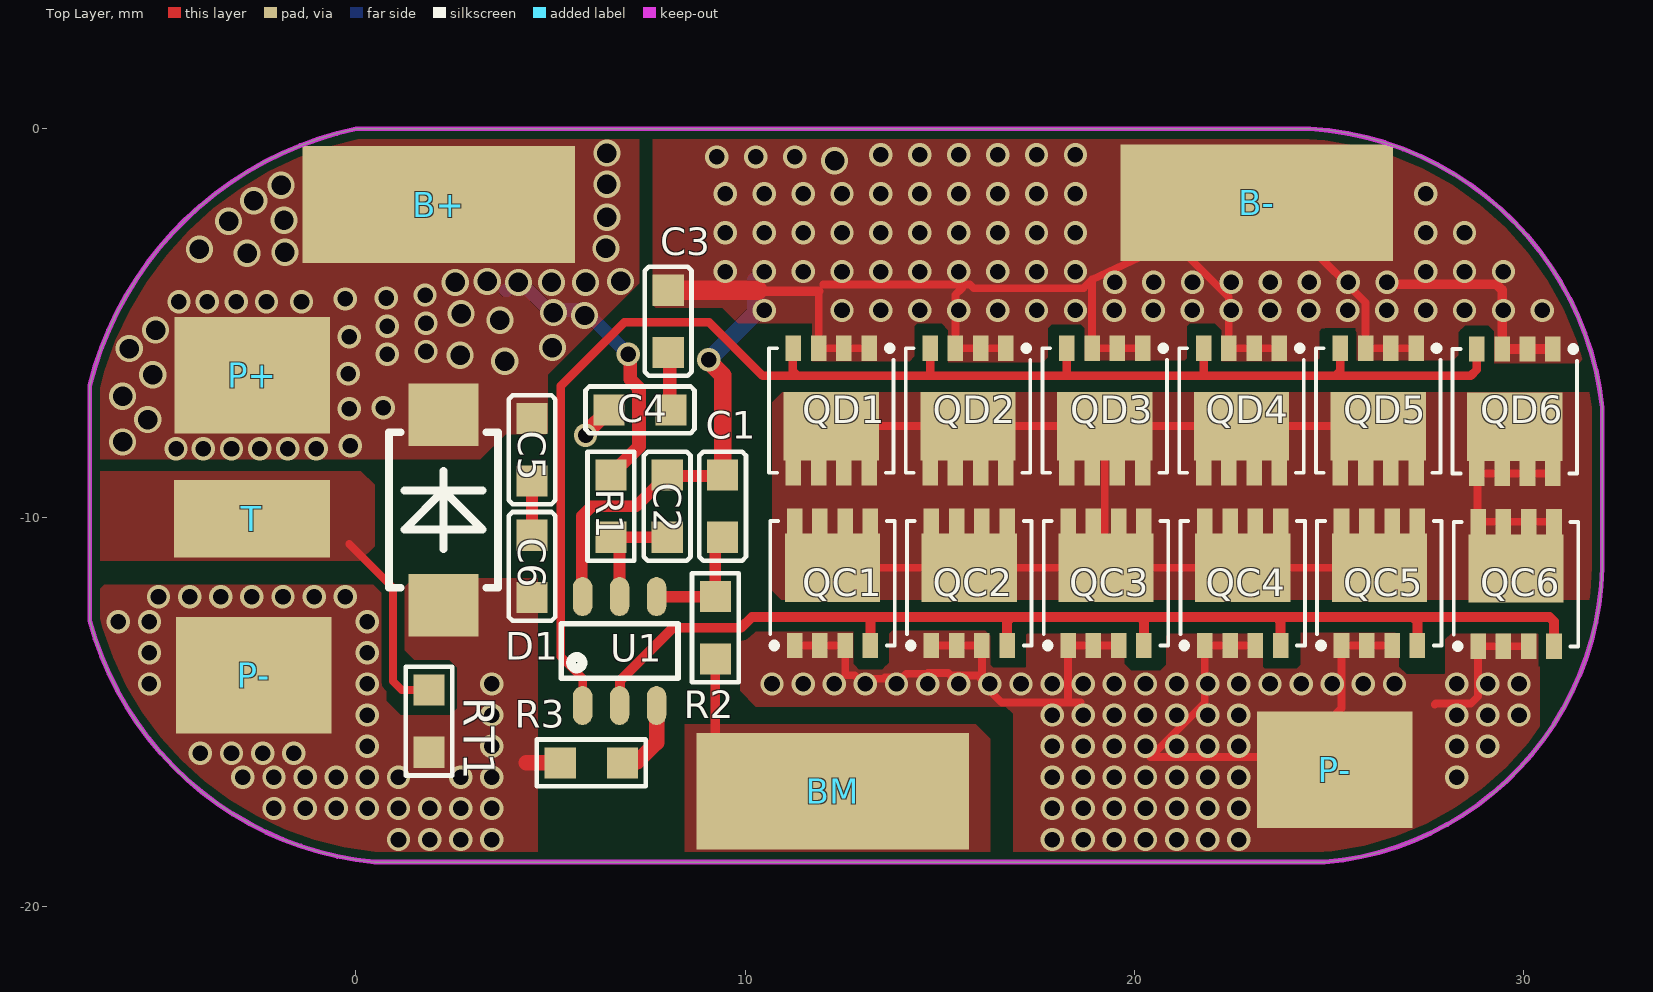
[diagram p0: Top Layer view]
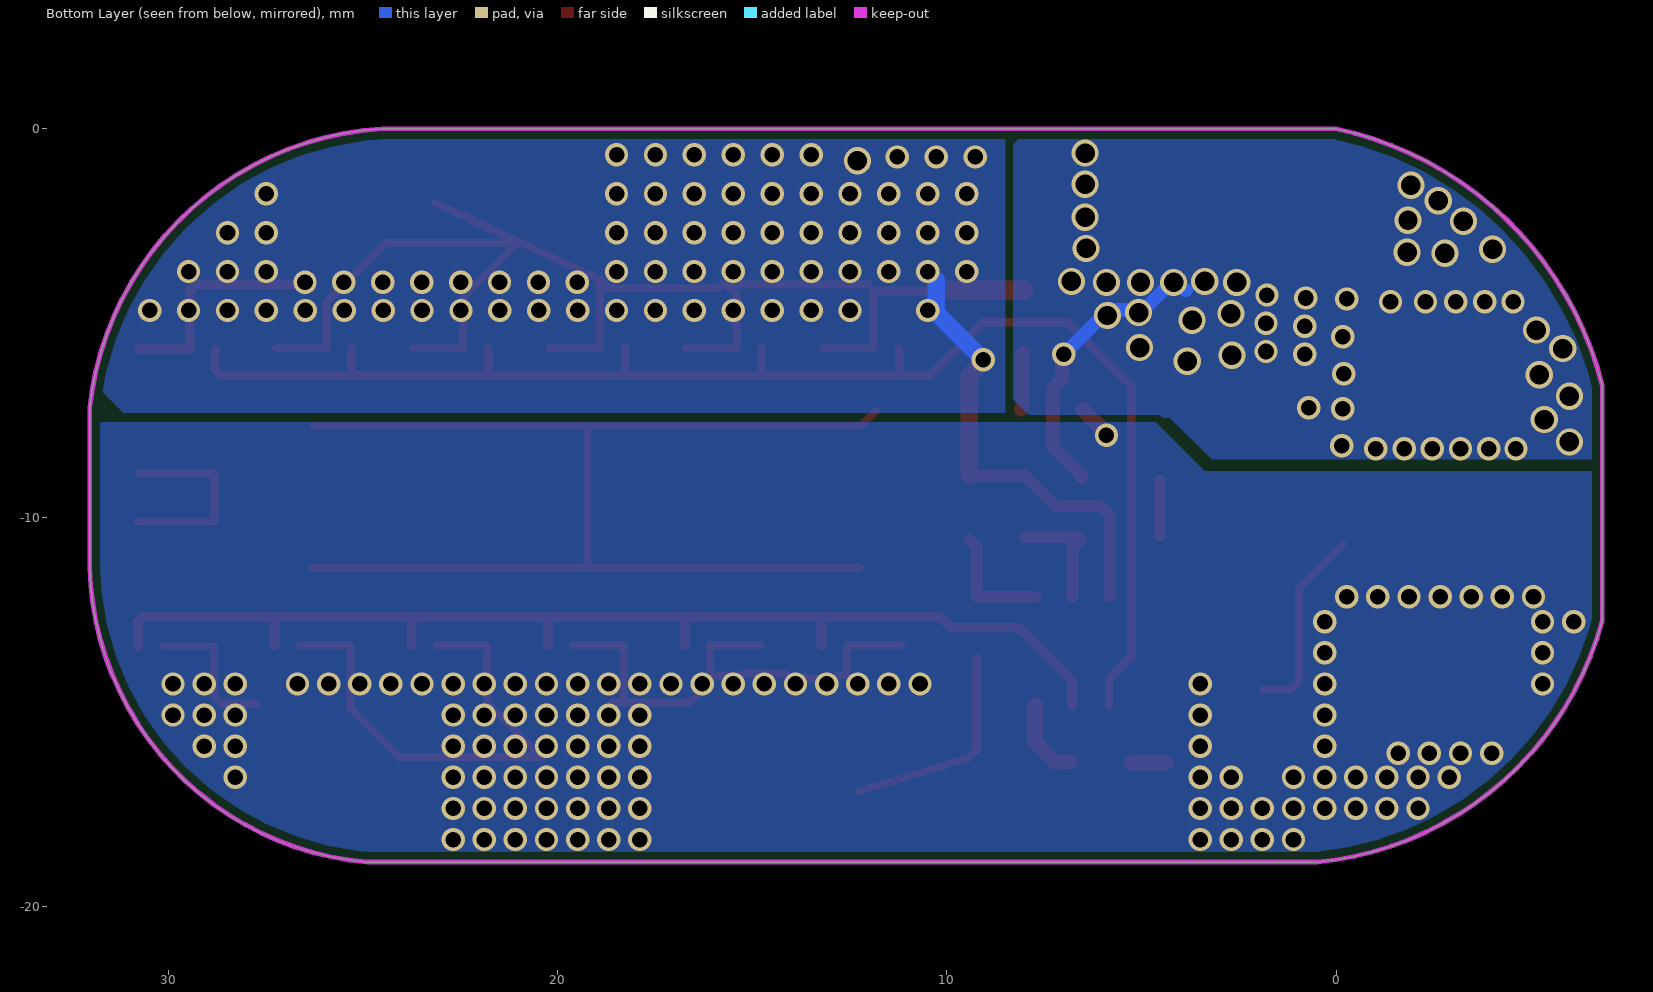
[diagram p1: Bottom Layer view, seen from below]
# Altium PCB MISC82114.PcbDoc
Units mm, origin at the board's own origin, x right, y up, seen from the top; angles counter-clockwise.
Board outline 38.88 x 18.85 mm, 2 copper layers (Top Layer, Bottom Layer); 31 components, 13 nets, 159 pads, 238 vias.

## Layer stack, top to bottom (the 12.6 mil dielectric is the usual default, probably not edited)
Top Solder: solder mask 0.0102, Solder Resist, Dk 3.5
Top Layer: signal copper 0.0356
Dielectric 1: dielectric 0.32, FR-4, Dk 4.8
Bottom Layer: signal copper 0.0356
Bottom Solder: solder mask 0.0102, Solder Resist, Dk 3.5

## Board outline
-6.843,-12.648 -6.843,-6.598 cw(c1.864,-8.781) 0,0 24.524,0 cw(c24.028,-8.037) 32.033,-7.161 32.033,-11.284 cw(c24.237,-11.079) 24.9,-18.849 0.48,-18.849 cw(c1.292,-10.465)

## Design rules (kind name [scope] priority, off if disabled: settings)
Clearance [All] p1: gap=0.2 ignorepadtopadclearanceinfootprint=FALSE
ComponentClearance [All] p1: gap=0.2 collisioncheckmode=3 verticalgap=0.254 showdistances=FALSE
PolygonConnect [All] p1: connectstyle=Direct reliefconductorwidth=0.254 reliefentries=4 polygonreliefangle="90 Angle" airgapwidth=0.254
RoutingVias [All] p1: holewidth=0.3 width=0.5 viastyle="Through Hole" minholewidth=0.3 minwidth=0.5 maxholewidth=0.3 maxwidth=0.5
SolderMaskExpansion [All] p1: expansion=0.102 istentingtop=FALSE
SupplyNets "Schematic Supply Nets" [InNet('P-')] p1: voltage=0.000
Width [All] p1: maxlimit=1 minlimit=0.15 preferedwidth=0.2
29 further rules are at their usual default settings.

## Components (designator, comment, footprint, x,y, rotation, side; value= is the part's Value field where it differs from the comment)
B+ "Pad" Pad10X8mm#1 2.127,-1.95 r0 top locked
B- "Pad" Pad10X8mm#1 23.152,-1.9 r0 top locked
BM "Pad" Pad10X8mm#1 12.252,-17.025 r0 top locked
C1 "0.1uF" C0603A 9.425,-9.7 r270 top
C2 "0.1uF" C0603A 8,-9.7 r270 top
C3 "0.1uF" C0603A 8.025,-4.95 r90 top
C4 "0.1uF" C0603A 7.3,-7.225 r0 top
C5 "0.1uF" C0603A 4.525,-8.25 r270 top
C6 "0.1uF" C0603A 4.525,-11.25 r270 top
D1 "RS2M" SMA(DO-214AC) 2.25,-9.8 r0 top
P+ "Pad" Pad10X8mm#2 -2.667,-6.337 r0 top locked
P- "Pad" Pad10X8mm#2 -2.623,-14.05 r0 top locked
P- "Pad" Pad10X8mm#3 25.152,-16.475 r90 top locked
QC1 "N MOS*" DFN-3x3L8(T3P) 12.248,-11.683 r0 top
QC2 "N MOS*" DFN-3x3L8(T3P) 15.762,-11.683 r0 top
QC3 "N MOS*" DFN-3x3L8(T3P) 19.276,-11.683 r0 top
QC4 "N MOS*" DFN-3x3L8(T3P) 22.791,-11.683 r0 top
QC5 "N MOS*" DFN-3x3L8(T3P) 26.305,-11.683 r0 top
QC6 "N MOS*" DFN-3x3L8(T3P) 29.816,-11.703 r0 top
QD1 "N MOS*" DFN-3x3L8(T3P) 12.217,-7.242 r180 top
QD2 "N MOS*" DFN-3x3L8(T3P) 15.731,-7.242 r180 top
QD3 "N MOS*" DFN-3x3L8(T3P) 19.245,-7.242 r180 top
QD4 "N MOS*" DFN-3x3L8(T3P) 22.76,-7.242 r180 top
QD5 "N MOS*" DFN-3x3L8(T3P) 26.274,-7.242 r180 top
QD6 "N MOS*" DFN-3x3L8(T3P) 29.785,-7.262 r180 top
R1 "330R" R0603A 6.55,-9.7 r270 top
R2 "330R" R0603A 9.237,-12.825 r90 top
R3 "2.2K" R0603A 6.05,-16.3 r0 top
RT1 "10K" R0603A 1.875,-15.225 r90 top
T "Pad" Pad10X8mm#4 -2.673,-10.025 r90 top locked
U1 "CW1025*" SOT23-6A 6.775,-13.425 r90 top

## Footprints (in the part's own frame and the unit in brackets; to place one, negate y for a bottom-side part, rotate by r counter-clockwise, add the part's x,y. Pads: shape width x height; smd on the part's side, far side on the other; paste and mask are expansions set on the pad)
C0603A [mm] "贴片电容"
  rect 0.8x0.8 smd mask+0.08: 1(-0.8,0) 2(0.8,0)
  silkscreen extent -1.4,-0.6 1.4,0.6
DFN-3x3L8(T3P) [mm] "贴片MOS"
  rect 0.4x0.65 smd: 1(0.975,-1.6) 2(-0.975,-1.6) 2(-0.325,-1.6) 2(0.325,-1.6) 3(-0.975,1.6) 3(-0.325,1.6) 3(0.325,1.6) 3(0.975,1.6)
  rect 2.45x1.76 smd: 3(0,0.4)
  silkscreen extent -1.6,-1.6 1.6,1.6
Pad10X8mm#1 [mm]
  rect 7x3 smd: 1(0,0)
Pad10X8mm#2 [mm]
  rect 4x3 smd: 1(0,0)
Pad10X8mm#3 [mm]
  rect 3x4 smd: 1(0,0)
Pad10X8mm#4 [mm]
  rect 2x4 smd: 1(0,0)
R0603A [mm] "贴片电阻"
  rect 0.8x0.8 smd mask+0.08: 1(-0.8,0) 2(0.8,0)
  silkscreen extent -1.4,-0.6 1.4,0.6
SMA(DO-214AC) [mm] "贴片二极管"
  rect 1.8x1.6 smd: 1(0,2.45) 2(0,-2.45)
  silkscreen extent -1.4,-2 1.4,2
SOT23-6A [mm]
  oval 1x0.5 smd mask+0.05: 1(-1.4,0.95) 2(-1.4,0) 3(-1.4,-0.95) 4(1.4,-0.95) 5(1.4,0) 6(1.4,0.95)
  silkscreen extent -0.7,-1.5 0.7,1.5

## Part data
B+ B- BM P+ P- P- T: "Connection pad (non-through-hole)"
C1 C2 C3 C4 C5 C6: library part CAP, "SMD capacitor"
D1: "SMD diode"
QC1 QC2 QC3 QC4 QC5 QC6 QD1 QD2 QD3 QD4 QD5 QD6: "SMD MOSFET"
R1 R2 R3 RT1: library part RES, "SMD resistor"
U1: "1-2S battery protection IC"

## Free pads (board coordinates)
  round 0.064 on Keep-Out: 1(-6.843,-12.648) 1(-6.843,-12.648) 1(-6.843,-6.598) 1(-6.843,-6.598) 1(0,0) 1(0,0) 1(0.48,-18.849) 1(0.48,-18.849) 1(24.524,0) 1(24.524,0) 1(24.9,-18.849) 1(24.9,-18.849) 1(32.033,-11.284) 1(32.033,-11.284) 1(32.033,-7.161) 1(32.033,-7.161)

## Via types
v1: diameter 0.6, hole 0.4, Top Layer to Bottom Layer, tented both sides, 207 vias
v2: diameter 0.7, hole 0.5, Top Layer to Bottom Layer, tented both sides, 31 vias

## Nets (pads, with @x,y where several pads share a name; then routed paths per layer and width w, separated by ;. In a path a pad name is that pad's centre, name@x,y a point inside that pad or via, vN(x,y) a via of type N, cw(c..) or ccw(c..) an arc to the next point about the centre after c; other vN are vias at no path point)
B+: B+.1 C5.1 D1.1 P+.1 R1.1 | length 7.6
  Top Layer w0.35: R1.1@6.55,-8.95 R1.1 7.275,-8.175 7.275,-6.67 7.048,-6.443 7.048,-5.848 v1(7,-5.8)
  Bottom Layer w0.35: 3.85,-4.15 3.88,-4.15 4.08,-3.95 4.237,-3.95 4.929,-4.642 5.158,-4.642 5.174,-4.658 5.792,-4.658 5.825,-4.625 v1(7,-5.8)
  other v1: -4.625,-8.225 -3.925,-8.225 -3.2,-8.225 -2.475,-8.225 -1.75,-8.225 -1.025,-8.225 -0.15,-8.15 -0.175,-7.2 0.7,-7.175 -0.2,-6.3 0.8,-5.8 1.8,-5.725 -0.175,-5.35 0.8,-5.075 1.8,-5 -4.55,-4.45 -3.825,-4.45 -3.075,-4.45 -2.3,-4.45 -1.4,-4.45 -0.275,-4.375 0.775,-4.35 1.775,-4.275
  other v2: -6,-8.05 -5.35,-7.475 -6,-6.875 -5.225,-6.325 3.825,-5.975 2.675,-5.825 -5.825,-5.65 5.05,-5.625 -5.15,-5.175 3.7,-4.925 5.875,-4.8 2.7,-4.75 5.075,-4.725 2.55,-3.95 4.175,-3.95 5.025,-3.95 5.9,-3.95 3.375,-3.925 6.8,-3.925 -2.8,-3.2 -1.825,-3.175 -4.025,-3.1 6.425,-3.075 -3.275,-2.375 -1.85,-2.35 6.45,-2.275 -2.625,-1.85 -1.925,-1.45 6.45,-1.425 6.45,-0.625
B-: B-.1 C1.1 C2.1 C3.2 QD1.2 QD2.2 QD3.2 QD4.2 QD5.2 QD6.2 U1.6 | length 56.9
  Top Layer w0.2: 11.892,-4.175 11.892,-5.642 12.542,-5.642 QD1.2@13.192,-5.642 ; 12.009,-4 15.777,-4 15.877,-4.1 18.697,-4.1 18.92,-3.877 ; 15.577,-4.1 15.406,-4.271 15.406,-5.642 16.056,-5.642 QD2.2@16.706,-5.642 ; QD3.2@20.22,-5.642 19.57,-5.642 18.92,-5.642 18.92,-3.877 ; QD4.2@23.735,-5.642 23.085,-5.642 22.435,-5.642 22.435,-4.328 B-.1@21.035,-2.928 ; QD5.2@27.249,-5.642 26.599,-5.642 25.949,-5.642 25.949,-4.472 24.405,-2.928 B-.1@21.035,-2.928 ; 18.92,-3.877 B-.1 B-.1@21.035,-2.928
  Top Layer w0.25: 10.35,-4.175 11.892,-4.175 ; v1@26.527,-3.975 26.552,-4 29.314,-4 29.46,-4.147 29.46,-5.662 30.11,-5.662 QD6.2@30.76,-5.662
  Top Layer w0.3: U1.6 5.8,-12 5.8,-9.955 6.055,-9.7 7.2,-9.7 7.975,-8.925 C2.1@8.025,-8.925 ; C2.1 C2.1@8.025,-8.925 ; C1.1@9.4,-8.925 C2.1@8.025,-8.925 ; 10.325,-4.15 10.35,-4.175
  Top Layer w0.45: v1(9.063,-5.937) 9.063,-5.977 9.425,-6.339 C1.1
  Top Layer w0.5: C3.2 10.325,-4.15
  Bottom Layer w0.45: v1(9.063,-5.937) 10.275,-4.725 10.275,-3.9
  other v1: 10.492,-4.67 12.492,-4.67 13.492,-4.67 14.492,-4.67 15.492,-4.67 16.492,-4.67 17.492,-4.67 18.492,-4.67 19.492,-4.67 20.492,-4.67 21.492,-4.67 22.492,-4.67 23.492,-4.67 24.492,-4.67 25.492,-4.67 26.492,-4.67 27.492,-4.67 28.492,-4.67 29.492,-4.67 30.492,-4.67 19.5,-3.95 20.5,-3.95 21.5,-3.95 22.5,-3.95 23.5,-3.95 24.5,-3.95 25.5,-3.95 26.5,-3.95 9.492,-3.67 10.492,-3.67 11.492,-3.67 12.492,-3.67 13.492,-3.67 14.492,-3.67 15.492,-3.67 16.492,-3.67 17.492,-3.67 18.492,-3.67 27.492,-3.67 28.492,-3.67 29.492,-3.67 9.492,-2.67 10.492,-2.67 11.492,-2.67 12.492,-2.67 13.492,-2.67 14.492,-2.67 15.492,-2.67 16.492,-2.67 17.492,-2.67 18.492,-2.67 27.492,-2.67 28.492,-2.67 9.492,-1.67 10.492,-1.67 11.492,-1.67 12.492,-1.67 13.492,-1.67 14.492,-1.67 15.492,-1.67 16.492,-1.67 17.492,-1.67 18.492,-1.67 27.492,-1.67 9.275,-0.725 10.275,-0.725 11.275,-0.725 13.492,-0.67 14.492,-0.67 15.492,-0.67 16.492,-0.67 17.492,-0.67 18.492,-0.67
  other v2: 12.3,-0.825
BM: BM.1 R2.1 | length 5.6
  Top Layer w0.2: BM.1@9.237,-15.96 9.46,-16.184 BM.1
  Top Layer w0.25: BM.1@9.237,-15.96 R2.1
CO: QC1.1 QC2.1 QC3.1 QC4.1 QC5.1 QC6.1 U1.2 | length 29.8
  Top Layer w0.254: U1.2 6.786,-14.814 6.786,-14.189 8.15,-12.825 9.9,-12.825 10.175,-12.55 10.648,-12.55 16.852,-12.55 ; QC1.1 13.223,-12.575 ; QC2.1 16.737,-12.665 16.852,-12.55 ; QC3.1 20.251,-12.65 20.152,-12.55 ; QC4.1 23.766,-12.659 23.657,-12.55 ; QC5.1 27.28,-12.667 27.163,-12.55 ; QC6.1 30.791,-12.667 30.674,-12.55 27.163,-12.55 ; 16.852,-12.55 20.152,-12.55 ; 20.152,-12.55 23.657,-12.55 ; 23.657,-12.55 27.163,-12.55
DO: QD1.1 QD2.1 QD3.1 QD4.1 QD5.1 QD6.1 U1.1 | length 37.5
  Top Layer w0.22: U1.1 5.825,-14.125 5.265,-13.565 5.265,-6.611 6.901,-4.975 9.075,-4.975 10.45,-6.35 11.344,-6.35 ; QD1.1 11.227,-5.657 11.227,-6.233 11.344,-6.35 ; QD2.1 14.756,-6.321 14.727,-6.35 ; QD3.1 18.27,-6.344 18.277,-6.35 ; QD4.1 21.785,-6.333 21.802,-6.35 ; QD5.1 25.299,-6.233 25.182,-6.35 ; QD6.1 28.81,-6.192 28.652,-6.35 25.182,-6.35 ; 11.344,-6.35 14.727,-6.35 ; 14.727,-6.35 18.277,-6.35 ; 18.277,-6.35 21.802,-6.35 ; 21.802,-6.35 25.182,-6.35
NetC3_1: C3.1 C4.2 | length 1.5
  Top Layer w0.35: C3.1 8.063,-5.788 8.063,-7.188 C4.2
NetC5_2: C5.2 C6.1 | length 1.4
  Top Layer w0.3: C6.1 C5.2
NetQC1_3: QC1.3 QC2.3 QC3.3 QC4.3 QC5.3 QC6.3 QD1.3 QD2.3 QD3.3 QD4.3 QD5.3 QD6.3 | length 37.5
  Top Layer w0.2: QD1.3@11.825,-7.25 12.217,-7.642 15.731,-7.642 QD3.3@19.245,-7.642 ; QC1.3@12.248,-11.283 15.762,-11.283 QC3.3@19.276,-11.283 ; QD5.3@26.274,-7.642 22.76,-7.642 QD3.3@19.245,-7.642 ; QC5.3@26.305,-11.283 22.791,-11.283 QC3.3@19.276,-11.283 ; QD6.3@30.76,-8.862 30.11,-8.862 29.46,-8.862 28.81,-8.862 28.826,-8.878 28.826,-10.088 28.841,-10.103 29.491,-10.103 30.141,-10.103 QC6.3@30.791,-10.103 ; QD3.3@19.245,-7.642 19.245,-11.252 QC3.3@19.276,-11.283
P-: C4.1 C6.2 D1.2 P-.1 QC1.2 QC2.2 QC3.2 QC4.2 QC5.2 QC6.2 R3.1 RT1.1 | length 32
  Top Layer w0.2: QC1.2@11.173,-13.25 11.206,-13.283 11.273,-13.283 11.923,-13.283 12.573,-13.283 12.573,-14.016 12.601,-14.044 12.815,-14.044 12.921,-14.15 12.933,-14.138 13.564,-14.138 13.598,-14.105 13.838,-14.105 13.86,-14.083 14.07,-14.083 14.146,-14.006 14.643,-14.006 14.662,-14.025 14.7,-13.987 15.224,-13.987 15.287,-14.05 15.977,-14.05 16.087,-14.16 16.087,-13.283 15.437,-13.283 QC2.2@14.787,-13.283 ; v1@16.087,-14.235 16.602,-14.75 18.301,-14.75 ; QC3.2@18.301,-13.358 18.301,-14.75 ; QC3.2@18.301,-13.283 18.951,-13.283 QC3.2@19.601,-13.283 ; 18.627,-14.75 18.301,-14.75 ; QC4.2@21.816,-13.358 21.816,-14.75 20.416,-16.15 24.077,-16.15 25.33,-14.897 QC5.2@25.33,-13.358 ; QC4.2@21.816,-13.283 22.466,-13.283 QC4.2@23.116,-13.283 ; QC5.2@25.33,-13.283 25.98,-13.283 QC5.2@26.63,-13.283 ; 27.727,-14.8 27.752,-14.775 28.652,-14.775 28.841,-14.586 28.841,-13.303 29.491,-13.303 QC6.2@30.141,-13.303
  Top Layer w0.4: 4.375,-16.3 R3.1 ; v1(5.9,-7.875) 5.9,-7.825 C4.1
  other v1: 1.092,-18.27 1.892,-18.27 2.692,-18.27 3.492,-18.27 17.892,-18.27 18.692,-18.27 19.492,-18.27 20.292,-18.27 21.092,-18.27 21.892,-18.27 22.692,-18.27 -2.108,-17.47 -1.308,-17.47 -0.508,-17.47 0.292,-17.47 1.092,-17.47 1.892,-17.47 2.692,-17.47 3.492,-17.47 17.892,-17.47 18.692,-17.47 19.492,-17.47 20.292,-17.47 21.092,-17.47 21.892,-17.47 22.692,-17.47 -2.908,-16.67 -2.108,-16.67 -1.308,-16.67 -0.508,-16.67 0.292,-16.67 1.092,-16.67 2.692,-16.67 3.492,-16.67 17.892,-16.67 18.692,-16.67 19.492,-16.67 20.292,-16.67 21.092,-16.67 21.892,-16.67 22.692,-16.67 28.292,-16.67 -4,-16.05 -3.2,-16.05 -2.4,-16.05 -1.6,-16.05 0.292,-15.87 3.492,-15.87 17.892,-15.87 18.692,-15.87 19.492,-15.87 20.292,-15.87 21.092,-15.87 21.892,-15.87 22.692,-15.87 28.292,-15.87 29.092,-15.87 0.292,-15.07 3.492,-15.07 17.892,-15.07 18.692,-15.07 19.492,-15.07 20.292,-15.07 21.092,-15.07 21.892,-15.07 22.692,-15.07 28.292,-15.07 29.092,-15.07 29.892,-15.07 -5.308,-14.27 0.292,-14.27 3.492,-14.27 10.692,-14.27 11.492,-14.27 12.292,-14.27 13.092,-14.27 13.892,-14.27 14.692,-14.27 15.492,-14.27 16.292,-14.27 17.092,-14.27 17.892,-14.27 18.692,-14.27 19.492,-14.27 20.292,-14.27 21.092,-14.27 21.892,-14.27 22.692,-14.27 23.492,-14.27 24.292,-14.27 25.092,-14.27 25.892,-14.27 26.692,-14.27 28.292,-14.27 29.092,-14.27 29.892,-14.27 -5.308,-13.47 0.292,-13.47 -6.108,-12.67 -5.308,-12.67 0.292,-12.67 -5.075,-12.025 -4.275,-12.025 -3.475,-12.025 -2.675,-12.025 -1.875,-12.025 -1.075,-12.025 -0.275,-12.025
T: RT1.2 T.1 | length 5
  Top Layer w0.2: -0.175,-10.675 0.95,-11.8 0.95,-14.2 1.175,-14.425 RT1.2
VC1: C1.2 R2.2 U1.4 | length 3.1
  Top Layer w0.3: U1.4 R2.2 9.237,-10.738 C1.2@9.425,-10.55
VDD: C2.2 R1.2 U1.5 | length 3
  Top Layer w0.3: U1.5 6.775,-10.775 6.55,-10.55 6.6,-10.5 6.775,-10.5 C2.2
VM: R3.2 U1.3 | length 2
  Top Layer w0.4: R3.2@6.85,-16.275 7.225,-16.275 7.725,-15.775 U1.3

## Polygon pours and split planes (outlines as drawn)
B+ on Top Layer "NONET_L-01_P-001" (solid, remove dead copper, pour order 16): -6.575,-3.602 -6.575,-8.5 3.2,-8.5 3.85,-7.85 4.875,-7.85 4.925,-7.8 4.925,-6.327 7.275,-3.977 7.275,-0.025 7.025,0.225 -2.748,0.225
P- on Top Layer "NONET_L-01_P-001" (solid, remove dead copper, pour order 5): 10.15,-12.925 9.877,-13.198 9.877,-14.45 10.277,-14.85 16.702,-14.85 16.892,-15.04 16.892,-19.1 27.827,-19.1 28.577,-18.35 28.577,-14.175 28.427,-14.025 27.002,-14.025 26.802,-13.825 26.802,-13.025 26.827,-13 26.752,-12.95 24.277,-12.95 24.277,-13.775 24.177,-13.875 23.352,-13.875 23.302,-13.825 23.302,-12.975 20.902,-12.975 20.827,-13.05 20.827,-13.775 20.677,-13.925 19.927,-13.925 19.752,-13.75 19.752,-12.975 17.252,-12.975 17.227,-13 17.227,-13.825 17.202,-13.85 16.377,-13.85 16.302,-13.775 16.302,-13.025 16.177,-12.9 13.777,-12.9 13.702,-12.975 13.702,-13.725 13.527,-13.9 12.927,-13.9 12.777,-13.75 12.777,-12.925
B- on Top Layer "NONET_L-01_P-001" (solid, remove dead copper, pour order 11): 9.814,-5 9.414,-4.6 7.7,-4.6 7.625,-4.525 7.625,-0.2 12.277,-0.2 12.277,-4.625 11.902,-5
B- on Top Layer "NONET_L-01_P-001" (solid, remove dead copper, pour order 7): 29.352,-0.251 29.352,-4.2 28.327,-5.225 28.327,-5.825 28.202,-5.95 25.727,-5.95 25.727,-5.225 25.627,-5.125 24.827,-5.125 24.752,-5.2 24.752,-5.9 24.677,-5.975 22.252,-5.975 22.252,-5.175 22.077,-5 21.427,-5 21.352,-5.075 21.352,-5.9 21.302,-5.95 18.727,-5.95 18.727,-5.125 18.627,-5.025 17.877,-5.025 17.777,-5.125 17.777,-5.875 17.652,-6 15.227,-6 15.227,-5.175 15.052,-5 14.427,-5 14.352,-5.075 14.352,-5.85 14.227,-5.975 11.727,-5.975 11.727,-5.325 11.727,0.125 25.447,0.125
B- on Top Layer "NONET_L-01_P-001" (solid, remove dead copper, pour order 15): 30.702,-1.85 31.877,-3.025 31.877,-5.8 31.652,-6.025 29.252,-6.025 29.252,-5.2 29.102,-5.05 26.377,-5.05 25.902,-4.575 25.902,-1.925 25.977,-1.85 27.352,-1.85
P- on Top Layer "NONET_L-01_P-001" (solid, remove dead copper, pour order 20): 4.675,-19.15 4.55,-19.275 -2.123,-19.275 -7.048,-14.35 -7.048,-12.3 -6.473,-11.725 0.627,-11.725 0.777,-11.875 0.777,-14.7 1.152,-15.075 2.425,-15.075 2.6,-14.9 2.6,-13.85 2.4,-13.65 1.5,-13.65 1.2,-13.35 1.2,-11.825 1.475,-11.55 4.675,-11.55
P- on Top Layer "NONET_L-01_P-001" (solid, remove dead copper, pour order 3): -7.048,-12.3 -6.473,-11.725 0.627,-11.725 0.777,-11.875 0.777,-14.7 1.152,-15.075 2.202,-15.075 2.577,-15.45 2.577,-19.275 -2.123,-19.275 -7.048,-14.35
P- on Top Layer "NONET_L-01_P-001" (solid, remove dead copper, pour order 14): 30.377,-12.975 30.427,-13.025 30.427,-16.95 28.002,-19.375 24.752,-19.375 24.752,-14.825 25.552,-14.025 27.977,-14.025 28.002,-14 28.002,-13.125 28.152,-12.975 30.352,-12.975
NetQC1_3 on Top Layer "NONET_L-01_P-001" (solid, remove dead copper, pour order 6): 32.152,-12.1 10.925,-12.1 10.702,-11.877 10.702,-7.025 10.952,-6.775 32.152,-6.775
BM on Top Layer "NONET_L-01_P-001" (solid, remove dead copper, pour order 4): 8.45,-18.7 8.45,-15.3 15.927,-15.3 16.302,-15.675 16.302,-18.7
T on Top Layer "NONET_L-01_P-001" (solid, remove dead copper, pour order 2): -6.798,-8.8 0.127,-8.8 0.477,-9.15 0.477,-10.725 0.102,-11.1 -6.798,-11.1
P- on Bottom Layer "NONET_L-01_P-001" (solid, remove dead copper, pour order 8): 4.627,-7.55 32.1,-7.55 32.677,-8.127 32.677,-15.225 27.498,-18.975 -4.223,-18.975 -6.748,-16.45 -6.723,-16.425 -6.723,-8.8 3.377,-8.8
B+ on Bottom Layer "NONET_L-01_P-001" (solid, remove dead copper, pour order 18): 3.2,-8.5 4.275,-7.425 7.825,-7.425 8.325,-6.925 8.325,-0.425 8,-0.1 -4.425,-0.1 -7.198,-2.873 -7.198,-8.25 -6.948,-8.5
B- on Bottom Layer "NONET_L-01_P-001" (solid, remove dead copper, pour order 9): 8.5,-7.3 31.175,-7.3 32.452,-6.023 32.452,-3.85 28.527,0.075 8.5,0.075

## Keep-outs
Keep-Out Layer:
  lines w0.127: -6.843,-12.648 ccw(c1.292,-10.465) 0.48,-18.849 24.9,-18.849 ccw(c24.237,-11.079) 32.033,-11.284 32.033,-7.161 ccw(c24.028,-8.037) 24.524,0 11,0 0,0 ccw(c1.864,-8.781) -6.843,-6.598 -6.843,-12.648

## Silkscreen, mask and mechanical layers (free items; w line width, h text height)
Top Solder:
  rectangle: 11.927,-4.075 18.802,-0.775
  rectangle: 17.377,-18.1 22.527,-14.25